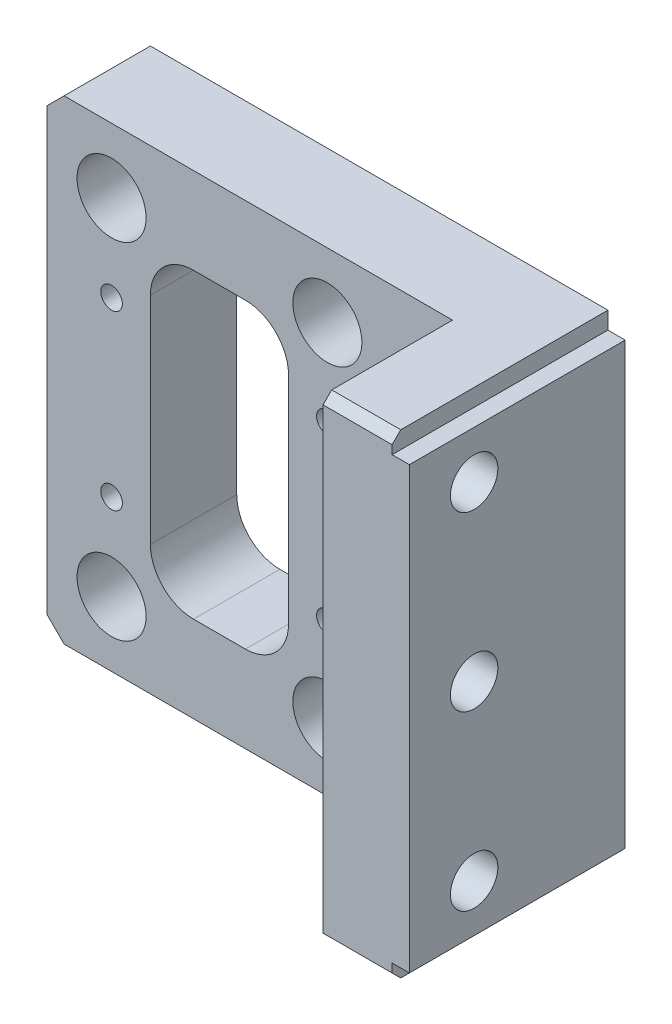
from build123d import *

# Parameters (mm, degrees)
SKETCH_1_W                = 57
SKETCH_1_H                = 55
EXTRUDE_1_DEPTH           = 10
SKETCH_2_W                = 16
SKETCH_2_H                = 35
CUT_EXTRUDE_1_DEPTH       = 41.847276531
HOLE_WIZARD_1_D           = 4.8
HOLE_WIZARD_1_CBORE_D     = 8
HOLE_WIZARD_1_CBORE_DEPTH = 6.6
HOLE_WIZARD_M3_1_D        = 2.5
FILLET_1_R                = 5
SKETCH_8_W                = 10
SKETCH_8_H                = 55
EXTRUDE_2_DEPTH           = 15
HOLE_WIZARD_2_D           = 5.5
HOLE_WIZARD_2_CBORE_D     = 10
HOLE_WIZARD_2_CBORE_DEPTH = 5.7
SKETCH_11_W               = 25
SKETCH_11_H               = 2
CUT_EXTRUDE_2_DEPTH       = 2
CHAMFER_3_SIZE            = 2
CHAMFER_4_SIZE            = 1


with BuildPart() as part:
    # 草图1 → 凸台-拉伸1 (new body)
    with BuildSketch(Plane.XY):
        Rectangle(SKETCH_1_W, SKETCH_1_H)
    extrude(amount=EXTRUDE_1_DEPTH)

    # 草图2 → 切除-拉伸1 (cut, through all)
    with BuildSketch(Plane.XY.offset(10)):
        with Locations((-8.5, 0)):
            Rectangle(SKETCH_2_W, SKETCH_2_H)
    extrude(amount=-CUT_EXTRUDE_1_DEPTH, mode=Mode.SUBTRACT)

    # 打孔尺寸(%根据)内六角圆柱头螺钉的类型1 (through all)
    with Locations(Plane.XY.offset(10)):
        with Locations((-21, 20), (4, 20), (-21, -20), (4, -20)):
            CounterBoreHole(HOLE_WIZARD_1_D / 2, HOLE_WIZARD_1_CBORE_D / 2, HOLE_WIZARD_1_CBORE_DEPTH)

    # M3 螺纹孔1 (through all)
    with Locations(Plane.XY.offset(10)):
        with Locations((-21, 10), (-21, -10), (4, 10), (4, -10)):
            Hole(HOLE_WIZARD_M3_1_D / 2)

    # 圆角1
    fillet_1_edges = [part.edges().sort_by_distance(p)[0] for p in [
        (-16.5, -17.5, 5),
        (-16.5, 17.5, 5),
        (-0.5, 17.5, 5),
        (-0.5, -17.5, 5),
    ]]
    fillet(fillet_1_edges, radius=FILLET_1_R)

    # 草图8 → 凸台-拉伸2 (add)
    with BuildSketch(Plane.XY.offset(10)):
        with Locations((23.5, 0)):
            Rectangle(SKETCH_8_W, SKETCH_8_H)
    extrude(amount=EXTRUDE_2_DEPTH)

    # 打孔尺寸(%根据)内六角圆柱头螺钉的类型2 (through all)
    with Locations(Plane.ZY.offset(-18.5)):
        with Locations((17.5, 20), (17.5, 0), (17.5, -20)):
            CounterBoreHole(HOLE_WIZARD_2_D / 2, HOLE_WIZARD_2_CBORE_D / 2, HOLE_WIZARD_2_CBORE_DEPTH)

    # 草图11 → 切除-拉伸2 (cut)
    with BuildSketch(Plane(origin=(28.5, 0, 0), x_dir=(0, 0, -1), z_dir=(1, 0, 0))):
        with Locations((-12.5, 26.5)):
            Rectangle(SKETCH_11_W, SKETCH_11_H)
        with Locations((-12.5, -26.5)):
            Rectangle(SKETCH_11_W, SKETCH_11_H)
    extrude(amount=-CUT_EXTRUDE_2_DEPTH, mode=Mode.SUBTRACT)

    # 倒角3
    chamfer_3_edges = [part.edges().sort_by_distance(p)[0] for p in [
        (-28.5, -27.5, 5),
        (-28.5, 27.5, 5),
    ]]
    chamfer(chamfer_3_edges, length=CHAMFER_3_SIZE)

    # 倒角4
    chamfer_4_edges = [part.edges().sort_by_distance(p)[0] for p in [
        (22.5, -27.5, 25),
        (22.5, 27.5, 25),
    ]]
    chamfer(chamfer_4_edges, length=CHAMFER_4_SIZE)


solid = part.part
